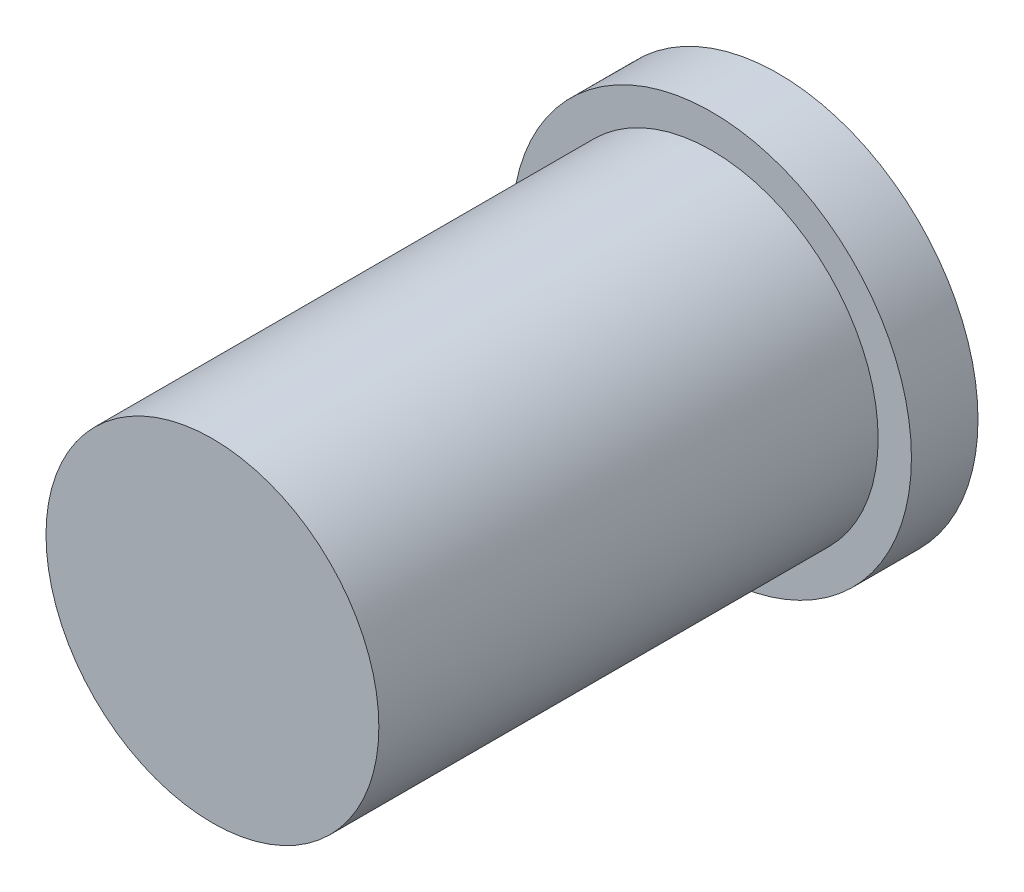
from build123d import *

# Parameters (mm, degrees)
SKETCH1_R           = 6
BOSS_EXTRUDE1_DEPTH = 2
SKETCH2_R           = 5
BOSS_EXTRUDE2_DEPTH = 15


with BuildPart() as part:
    # Sketch1 → Boss-Extrude1 (new body)
    with BuildSketch(Plane.XY):
        Circle(SKETCH1_R)
    extrude(amount=BOSS_EXTRUDE1_DEPTH)

    # Sketch2 → Boss-Extrude2 (add)
    with BuildSketch(Plane.XY.offset(2)):
        Circle(SKETCH2_R)
    extrude(amount=BOSS_EXTRUDE2_DEPTH)


solid = part.part
